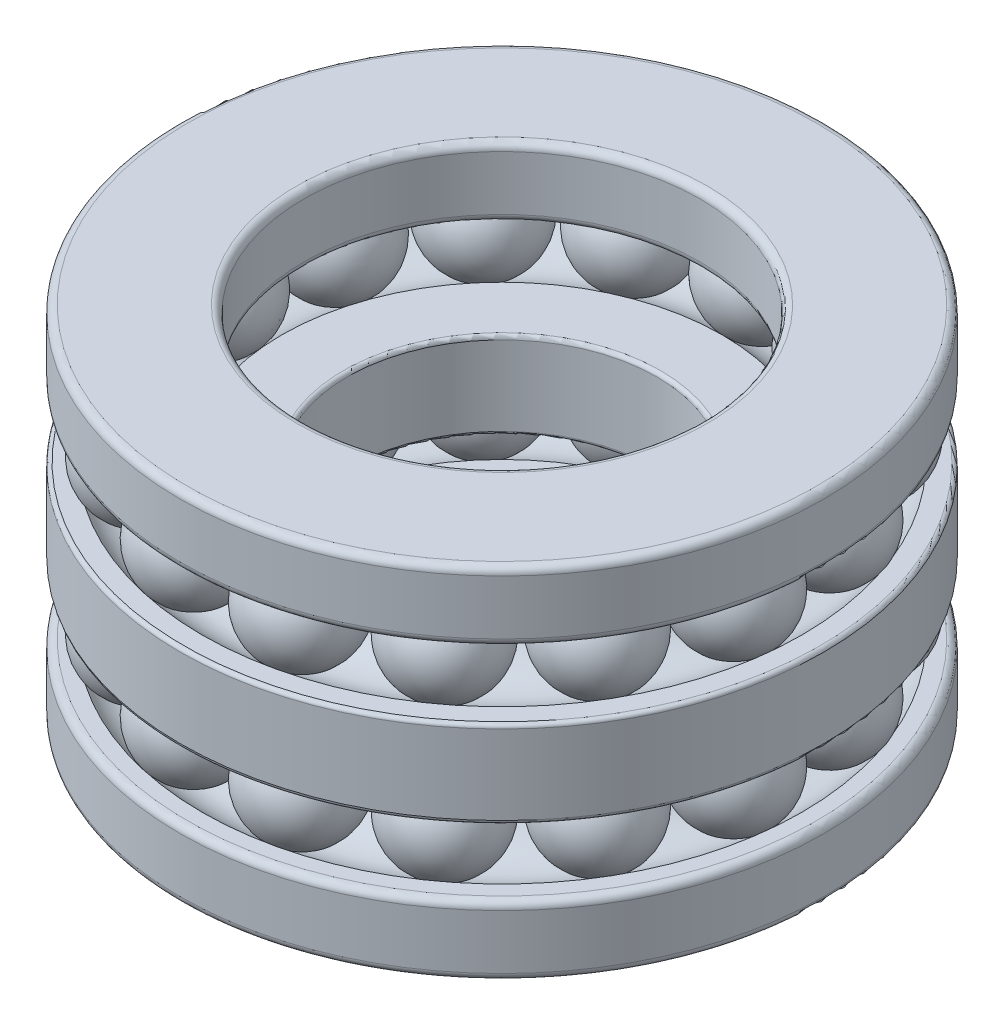
from build123d import *

# Parameters (mm, degrees)
CIRPATTERN5_COUNT = 15


with BuildPart() as part:
    # Sketch2 → Revolve1 (revolve)
    with BuildSketch(Plane(origin=(0, 0, 0), x_dir=(0, 0, -1), z_dir=(1, 0, 0))):
        with BuildLine():
            ThreePointArc((24.217141588, 8.9), (21, 10.4), (17.782858412, 8.9))
            Line((17.782858412, 8.9), (16.6, 8.9))
            ThreePointArc((16.6, 8.9), (16.175735931, 9.075735931), (16, 9.5))
            Line((16, 9.5), (16, 13.9))
            ThreePointArc((16, 13.9), (16.175735931, 14.324264069), (16.6, 14.5))
            Line((16.6, 14.5), (25.4, 14.5))
            ThreePointArc((25.4, 14.5), (25.824264069, 14.324264069), (26, 13.9))
            Line((26, 13.9), (26, 9.5))
            ThreePointArc((26, 9.5), (25.824264069, 9.075735931), (25.4, 8.9))
            Line((25.4, 8.9), (24.217141588, 8.9))
        make_face()
        with BuildLine():
            ThreePointArc((17.782858412, 3.5), (21, 2), (24.217141588, 3.5))
            Line((24.217141588, 3.5), (25.7, 3.5))
            ThreePointArc((25.7, 3.5), (25.912132034, 3.412132034), (26, 3.2))
            Line((26, 3.2), (26, -3.2))
            ThreePointArc((26, -3.2), (25.912132034, -3.412132034), (25.7, -3.5))
            Line((25.7, -3.5), (24.217141588, -3.5))
            ThreePointArc((24.217141588, -3.5), (21, -2), (17.782858412, -3.5))
            Line((17.782858412, -3.5), (12.8, -3.5))
            ThreePointArc((12.8, -3.5), (12.587867966, -3.412132034), (12.5, -3.2))
            Line((12.5, -3.2), (12.5, 3.2))
            ThreePointArc((12.5, 3.2), (12.587867966, 3.412132034), (12.8, 3.5))
            Line((12.8, 3.5), (17.782858412, 3.5))
        make_face()
        with BuildLine():
            ThreePointArc((17.782858412, -8.9), (21, -10.4), (24.217141588, -8.9))
            Line((24.217141588, -8.9), (25.4, -8.9))
            ThreePointArc((25.4, -8.9), (25.824264069, -9.075735931), (26, -9.5))
            Line((26, -9.5), (26, -13.9))
            ThreePointArc((26, -13.9), (25.824264069, -14.324264069), (25.4, -14.5))
            Line((25.4, -14.5), (16.6, -14.5))
            ThreePointArc((16.6, -14.5), (16.175735931, -14.324264069), (16, -13.9))
            Line((16, -13.9), (16, -9.5))
            ThreePointArc((16, -9.5), (16.175735931, -9.075735931), (16.6, -8.9))
            Line((16.6, -8.9), (17.782858412, -8.9))
        make_face()
    revolve(axis=Axis((0, 0, 0), (0, 1, 0)))


with BuildPart() as body_2:
    # Sketch3 → Revolve2 (revolve)
    with BuildSketch(Plane(origin=(0, 0, 0), x_dir=(0, 0, -1), z_dir=(1, 0, 0))):
        with BuildLine():
            ThreePointArc((21, 2), (25.2, 6.2), (21, 10.4))
            Line((21, 10.4), (21, 2))
        make_face()
        with BuildLine():
            ThreePointArc((21, -10.4), (25.2, -6.2), (21, -2))
            Line((21, -2), (21, -10.4))
        make_face()
    revolve(axis=Axis((0, 10.4, -21), (0, -1, 0)))


with BuildPart() as cirpattern5_1:
    # CirPattern5: pattern copy
    add(body_2.part.rotate(Axis((0, 0, 0), (0, 1, 0)), 1 * 360 / CIRPATTERN5_COUNT))


with BuildPart() as cirpattern5_2:
    # CirPattern5: pattern copy
    add(body_2.part.rotate(Axis((0, 0, 0), (0, 1, 0)), 2 * 360 / CIRPATTERN5_COUNT))


with BuildPart() as cirpattern5_3:
    # CirPattern5: pattern copy
    add(body_2.part.rotate(Axis((0, 0, 0), (0, 1, 0)), 3 * 360 / CIRPATTERN5_COUNT))


with BuildPart() as cirpattern5_4:
    # CirPattern5: pattern copy
    add(body_2.part.rotate(Axis((0, 0, 0), (0, 1, 0)), 4 * 360 / CIRPATTERN5_COUNT))


with BuildPart() as cirpattern5_5:
    # CirPattern5: pattern copy
    add(body_2.part.rotate(Axis((0, 0, 0), (0, 1, 0)), 5 * 360 / CIRPATTERN5_COUNT))


with BuildPart() as cirpattern5_6:
    # CirPattern5: pattern copy
    add(body_2.part.rotate(Axis((0, 0, 0), (0, 1, 0)), 6 * 360 / CIRPATTERN5_COUNT))


with BuildPart() as cirpattern5_7:
    # CirPattern5: pattern copy
    add(body_2.part.rotate(Axis((0, 0, 0), (0, 1, 0)), 7 * 360 / CIRPATTERN5_COUNT))


with BuildPart() as cirpattern5_8:
    # CirPattern5: pattern copy
    add(body_2.part.rotate(Axis((0, 0, 0), (0, 1, 0)), 8 * 360 / CIRPATTERN5_COUNT))


with BuildPart() as cirpattern5_9:
    # CirPattern5: pattern copy
    add(body_2.part.rotate(Axis((0, 0, 0), (0, 1, 0)), 9 * 360 / CIRPATTERN5_COUNT))


with BuildPart() as cirpattern5_10:
    # CirPattern5: pattern copy
    add(body_2.part.rotate(Axis((0, 0, 0), (0, 1, 0)), 10 * 360 / CIRPATTERN5_COUNT))


with BuildPart() as cirpattern5_11:
    # CirPattern5: pattern copy
    add(body_2.part.rotate(Axis((0, 0, 0), (0, 1, 0)), 11 * 360 / CIRPATTERN5_COUNT))


with BuildPart() as cirpattern5_12:
    # CirPattern5: pattern copy
    add(body_2.part.rotate(Axis((0, 0, 0), (0, 1, 0)), 12 * 360 / CIRPATTERN5_COUNT))


with BuildPart() as cirpattern5_13:
    # CirPattern5: pattern copy
    add(body_2.part.rotate(Axis((0, 0, 0), (0, 1, 0)), 13 * 360 / CIRPATTERN5_COUNT))


with BuildPart() as cirpattern5_14:
    # CirPattern5: pattern copy
    add(body_2.part.rotate(Axis((0, 0, 0), (0, 1, 0)), 14 * 360 / CIRPATTERN5_COUNT))


solid = Compound([part.part, body_2.part, cirpattern5_1.part, cirpattern5_2.part, cirpattern5_3.part, cirpattern5_4.part, cirpattern5_5.part, cirpattern5_6.part, cirpattern5_7.part, cirpattern5_8.part, cirpattern5_9.part, cirpattern5_10.part, cirpattern5_11.part, cirpattern5_12.part, cirpattern5_13.part, cirpattern5_14.part])
